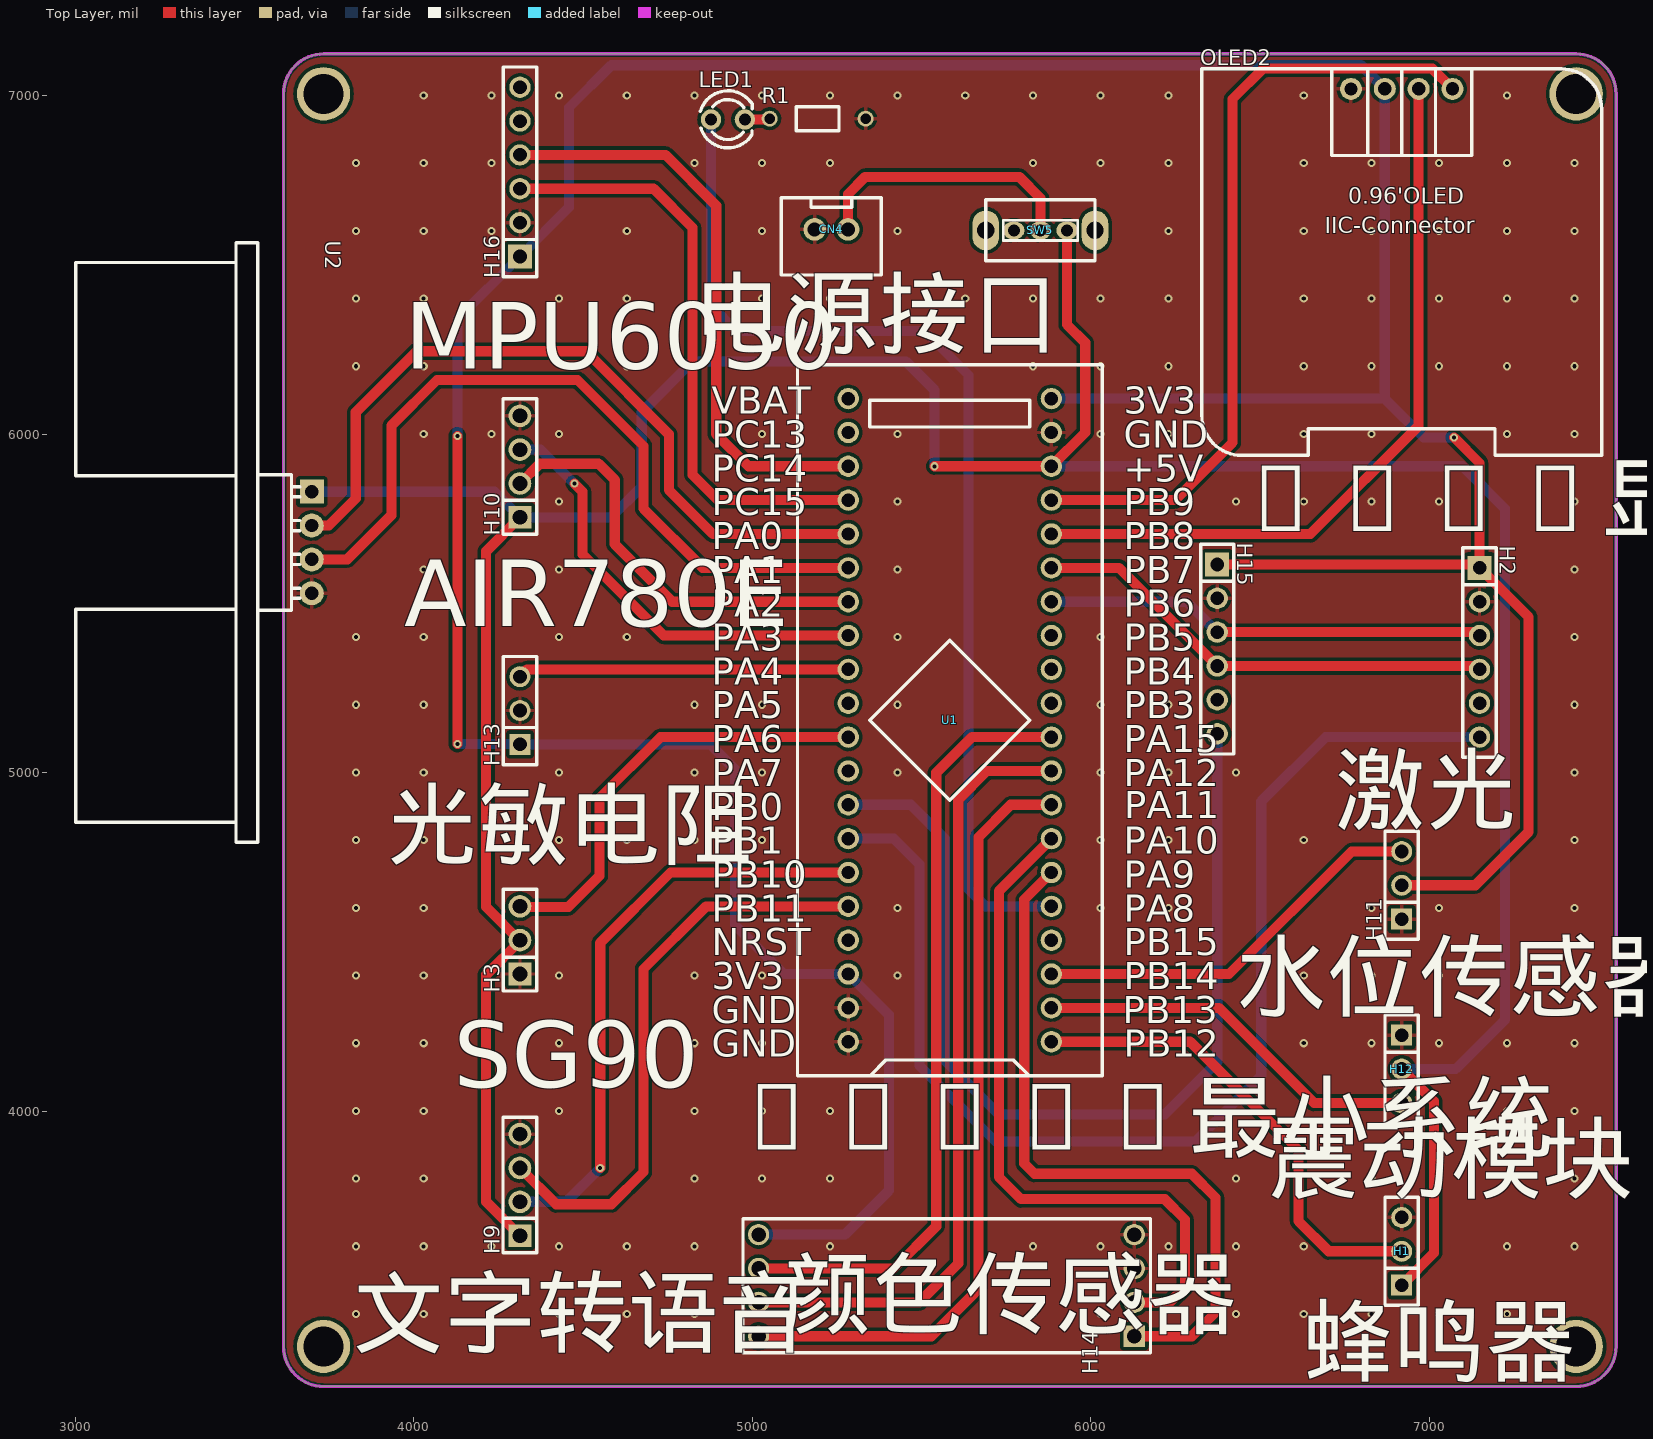
[diagram p0: Top Layer view]
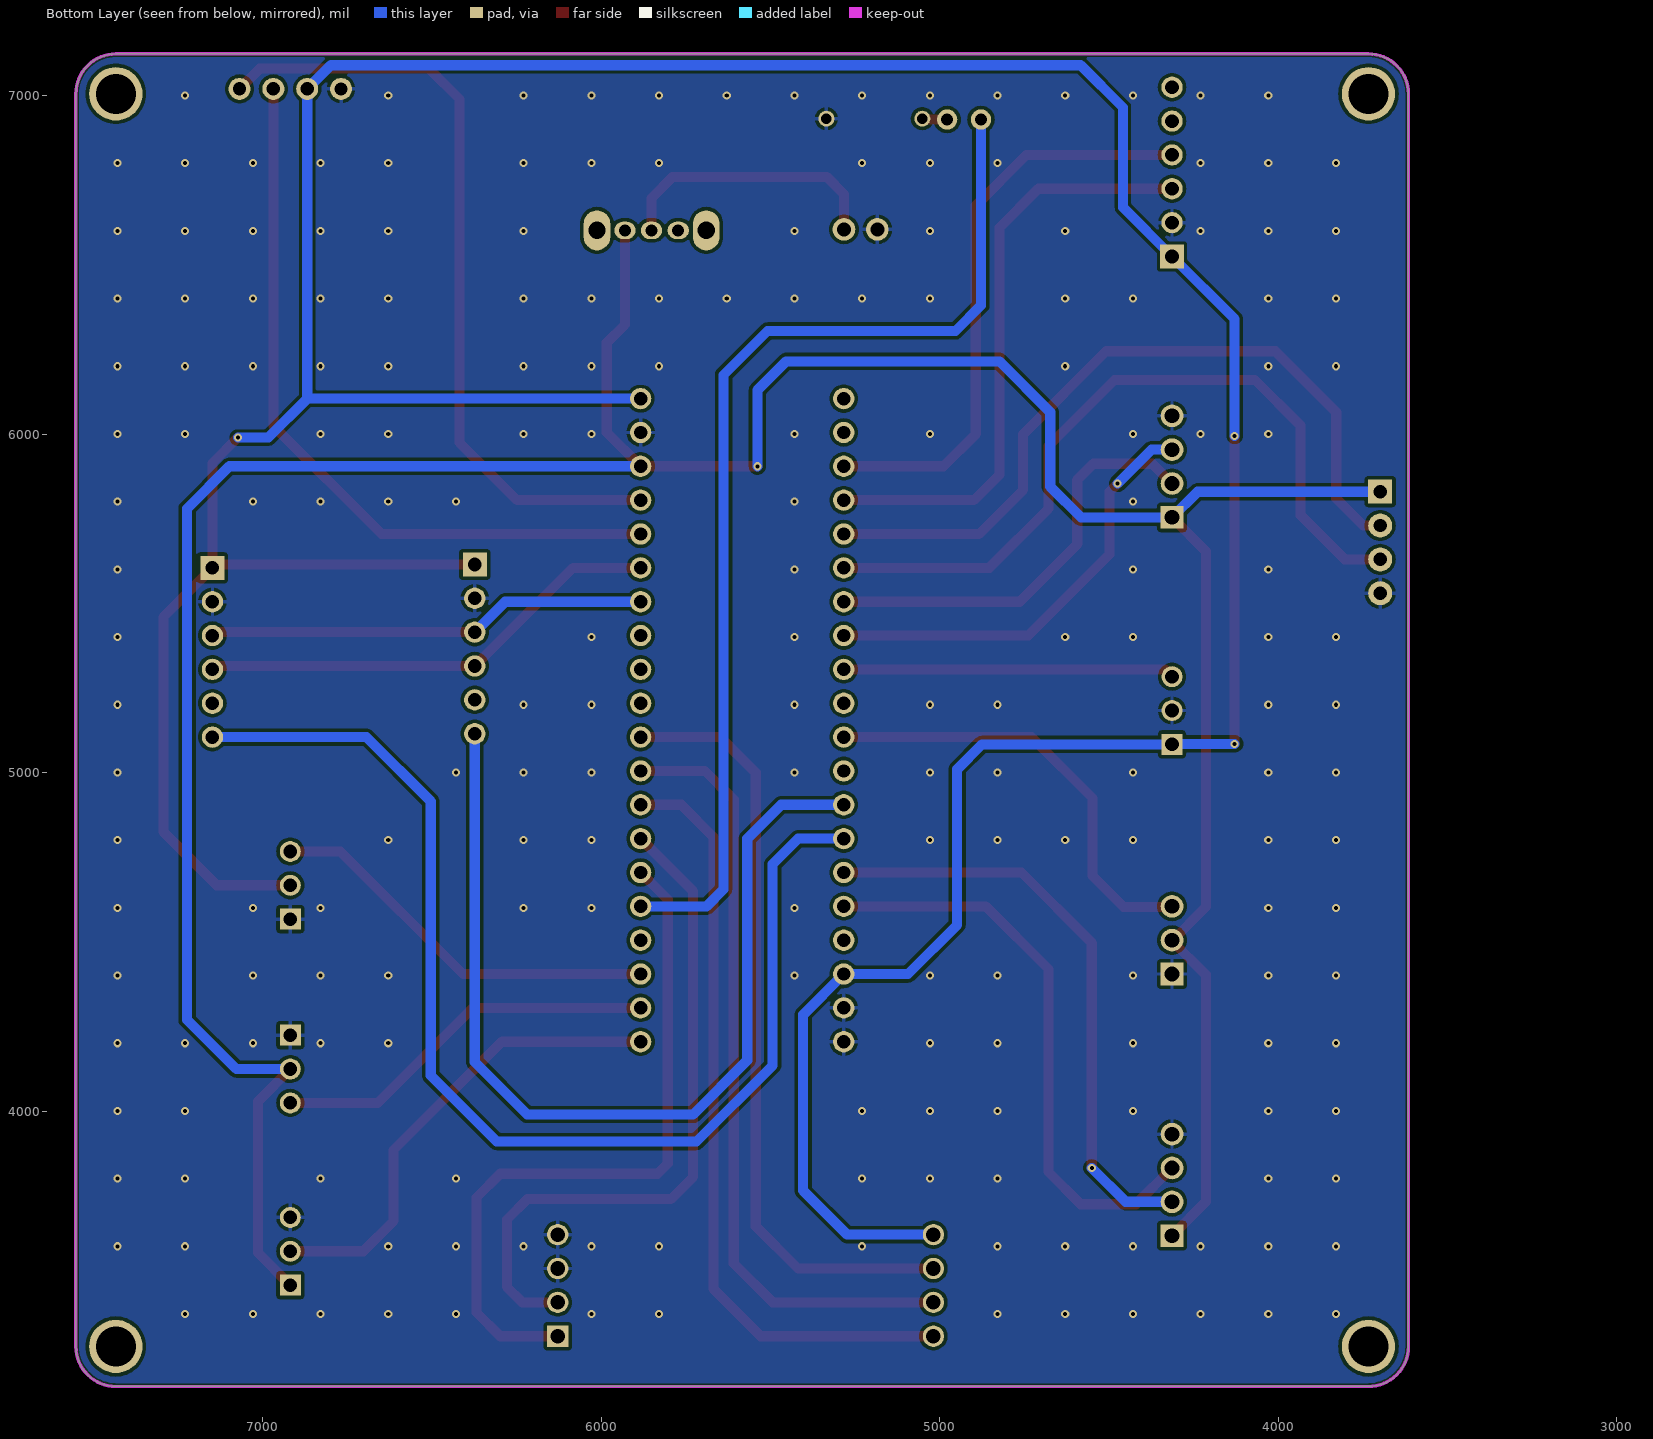
[diagram p1: Bottom Layer view, seen from below]
# Altium PCB MISC51292.pcbdoc
Units mil, origin at the board's own origin, x right, y up, seen from the top; angles counter-clockwise.
Board outline 3937.01 x 3937.01 mil, 2 copper layers (Top Layer, Bottom Layer), stack 62.206 mil thick; 18 components, 39 nets, 112 pads, 202 vias.

## Layer stack, top to bottom
Top Solder Mask Layer: solder mask 0.394, Dk 3.3
Top Layer: signal copper 1.379
Dielectric1: surface 59.449, FR4, Dk 4.5
Bottom Layer: signal copper 1.378
Bottom Solder Mask Layer: solder mask 0.394, Dk 3.3

## Board outline
3733.82,7123.5 ccw(c3733.82,7005.39) 3615.71,7005.39 3615.71,3304.61 ccw(c3733.82,3304.61) 3733.82,3186.5 7434.61,3186.5 ccw(c7434.61,3304.61) 7552.72,3304.61 7552.72,7005.39 ccw(c7434.61,7005.39) 7434.61,7123.5 3733.82,7123.5

## Design rules (kind name [scope] priority, off if disabled: settings)
BoardOutlineClearance copperThickness2oz_1 [All] p2 off: genericclearance=7.99 ignorepadtopadclearanceinfootprint=FALSE except(0: Arc-SplitContinuation Track-SplitContinuation SMDPad-SplitContinuation THPad-SplitContinuation Via-SplitContinuation Fill-SplitContinuation Region-SplitContinuation Poly-SplitContinuation Text-SplitContinuation Hole-SplitContinuation; 5.98: Arc-CutoutEdge Track-CutoutEdge SMDPad-CutoutEdge THPad-CutoutEdge Via-CutoutEdge Text-CutoutEdge; 6.9: Hole-OutlineEdge Hole-CutoutEdge; 10: Poly-OutlineEdge Poly-CutoutEdge; 11.81: Arc-OutlineEdge Track-OutlineEdge SMDPad-OutlineEdge THPad-OutlineEdge Via-OutlineEdge Fill-OutlineEdge Region-OutlineEdge Text-OutlineEdge Fill-CutoutEdge Region-CutoutEdge)
BoardOutlineClearance Plane_innerPlane_1 [All] p4 off: genericclearance=4.02 ignorepadtopadclearanceinfootprint=FALSE except(0: Arc-SplitContinuation Track-SplitContinuation SMDPad-SplitContinuation THPad-SplitContinuation Via-SplitContinuation Fill-SplitContinuation Region-SplitContinuation Poly-SplitContinuation Text-SplitContinuation Hole-SplitContinuation; 5.98: Arc-CutoutEdge Track-CutoutEdge SMDPad-CutoutEdge THPad-CutoutEdge Via-CutoutEdge Text-CutoutEdge; 6.9: Hole-OutlineEdge Hole-CutoutEdge; 10: Poly-OutlineEdge Poly-CutoutEdge; 11.81: Arc-OutlineEdge Track-OutlineEdge SMDPad-OutlineEdge THPad-OutlineEdge Via-OutlineEdge Fill-OutlineEdge Region-OutlineEdge Text-OutlineEdge Fill-CutoutEdge Region-CutoutEdge)
BoardOutlineClearance Copper_copperRegion_1 [All] p6 off: genericclearance=4.02 ignorepadtopadclearanceinfootprint=FALSE except(0: Arc-SplitContinuation Track-SplitContinuation SMDPad-SplitContinuation THPad-SplitContinuation Via-SplitContinuation Fill-SplitContinuation Region-SplitContinuation Poly-SplitContinuation Text-SplitContinuation Hole-SplitContinuation; 5.98: Arc-CutoutEdge Track-CutoutEdge SMDPad-CutoutEdge THPad-CutoutEdge Via-CutoutEdge Text-CutoutEdge; 6.9: Hole-OutlineEdge Hole-CutoutEdge; 10: Poly-OutlineEdge Poly-CutoutEdge; 11.81: Arc-OutlineEdge Track-OutlineEdge SMDPad-OutlineEdge THPad-OutlineEdge Via-OutlineEdge Fill-OutlineEdge Region-OutlineEdge Text-OutlineEdge Fill-CutoutEdge Region-CutoutEdge)
BoardOutlineClearance Copper_copperRegion_copperThickness1oz_1 [All] p8 off: genericclearance=4.02 ignorepadtopadclearanceinfootprint=FALSE except(0: Arc-SplitContinuation Track-SplitContinuation SMDPad-SplitContinuation THPad-SplitContinuation Via-SplitContinuation Fill-SplitContinuation Region-SplitContinuation Poly-SplitContinuation Text-SplitContinuation Hole-SplitContinuation; 5.98: Arc-CutoutEdge Track-CutoutEdge SMDPad-CutoutEdge THPad-CutoutEdge Via-CutoutEdge Text-CutoutEdge; 6.9: Hole-OutlineEdge Hole-CutoutEdge; 10: Poly-OutlineEdge Poly-CutoutEdge; 11.81: Arc-OutlineEdge Track-OutlineEdge SMDPad-OutlineEdge THPad-OutlineEdge Via-OutlineEdge Fill-OutlineEdge Region-OutlineEdge Text-OutlineEdge Fill-CutoutEdge Region-CutoutEdge)
BoardOutlineClearance Copper_copperRegion_Copper_copperRegion_1 [All] p10 off: genericclearance=4.02 ignorepadtopadclearanceinfootprint=FALSE except(0: Arc-SplitContinuation Track-SplitContinuation SMDPad-SplitContinuation THPad-SplitContinuation Via-SplitContinuation Fill-SplitContinuation Region-SplitContinuation Poly-SplitContinuation Text-SplitContinuation Hole-SplitContinuation; 5.98: Arc-CutoutEdge Track-CutoutEdge SMDPad-CutoutEdge THPad-CutoutEdge Via-CutoutEdge Text-CutoutEdge; 6.9: Hole-OutlineEdge Hole-CutoutEdge; 10: Poly-OutlineEdge Poly-CutoutEdge; 11.81: Arc-OutlineEdge Track-OutlineEdge SMDPad-OutlineEdge THPad-OutlineEdge Via-OutlineEdge Fill-OutlineEdge Region-OutlineEdge Text-OutlineEdge Fill-CutoutEdge Region-CutoutEdge)
BoardOutlineClearance copperThickness1oz_1 [All] p12: genericclearance=4.02 ignorepadtopadclearanceinfootprint=FALSE except(0: Arc-SplitContinuation Track-SplitContinuation SMDPad-SplitContinuation THPad-SplitContinuation Via-SplitContinuation Fill-SplitContinuation Region-SplitContinuation Poly-SplitContinuation Text-SplitContinuation Hole-SplitContinuation; 5.98: Arc-CutoutEdge Track-CutoutEdge SMDPad-CutoutEdge THPad-CutoutEdge Via-CutoutEdge Text-CutoutEdge; 6.9: Hole-OutlineEdge Hole-CutoutEdge; 10: Poly-OutlineEdge Poly-CutoutEdge; 11.81: Arc-OutlineEdge Track-OutlineEdge SMDPad-OutlineEdge THPad-OutlineEdge Via-OutlineEdge Fill-OutlineEdge Region-OutlineEdge Text-OutlineEdge Fill-CutoutEdge Region-CutoutEdge)
Clearance copperThickness2oz [All] p1 off: gap=7.99 ignorepadtopadclearanceinfootprint=FALSE except(5.98: SMDPad-Track SMDPad-SMDPad THPad-Track SMDPad-THPad THPad-THPad Track-Via SMDPad-Via THPad-Via Via-Via Fill-SMDPad Region-SMDPad Fill-THPad Region-THPad Fill-Via Region-Via Fill-Fill Fill-Region Region-Region Arc-Track Arc-SMDPad Arc-THPad Arc-Via Fill-Arc Region-Arc Arc-Arc Text-Track SMDPad-Text Text-THPad Text-Via Fill-Text Region-Text Arc-Text Text-Text; 6.9: Hole-Track Hole-SMDPad Hole-THPad Hole-Via Fill-Hole Region-Hole Hole-Arc Hole-Text; 10: Poly-Track Poly-SMDPad Poly-THPad Poly-Via Poly-Fill Poly-Region Poly-Poly Poly-Arc Poly-Text Poly-Hole; 11.81: Fill-Track Region-Track)
Clearance Plane_innerPlane [All] p3 off: gap=4.02 ignorepadtopadclearanceinfootprint=FALSE except(5.98: SMDPad-Track SMDPad-SMDPad THPad-Track SMDPad-THPad THPad-THPad Track-Via SMDPad-Via THPad-Via Via-Via Fill-SMDPad Region-SMDPad Fill-THPad Region-THPad Fill-Via Region-Via Fill-Fill Fill-Region Region-Region Arc-Track Arc-SMDPad Arc-THPad Arc-Via Fill-Arc Region-Arc Arc-Arc Text-Track SMDPad-Text Text-THPad Text-Via Fill-Text Region-Text Arc-Text Text-Text; 6.9: Hole-Track Hole-SMDPad Hole-THPad Hole-Via Fill-Hole Region-Hole Hole-Arc Hole-Text; 10: Poly-Track Poly-SMDPad Poly-THPad Poly-Via Poly-Fill Poly-Region Poly-Poly Poly-Arc Poly-Text Poly-Hole; 11.81: Fill-Track Region-Track)
Clearance Copper_copperRegion [All] p5 off: gap=4.02 ignorepadtopadclearanceinfootprint=FALSE except(5.98: SMDPad-Track SMDPad-SMDPad THPad-Track SMDPad-THPad THPad-THPad Track-Via SMDPad-Via THPad-Via Via-Via Fill-SMDPad Region-SMDPad Fill-THPad Region-THPad Fill-Via Region-Via Fill-Fill Fill-Region Region-Region Arc-Track Arc-SMDPad Arc-THPad Arc-Via Fill-Arc Region-Arc Arc-Arc Text-Track SMDPad-Text Text-THPad Text-Via Fill-Text Region-Text Arc-Text Text-Text; 6.9: Hole-Track Hole-SMDPad Hole-THPad Hole-Via Fill-Hole Region-Hole Hole-Arc Hole-Text; 10: Poly-Track Poly-SMDPad Poly-THPad Poly-Via Poly-Fill Poly-Region Poly-Poly Poly-Arc Poly-Text Poly-Hole; 11.81: Fill-Track Region-Track)
Clearance Copper_copperRegion_copperThickness1oz [All] p7 off: gap=4.02 ignorepadtopadclearanceinfootprint=FALSE except(5.98: SMDPad-Track SMDPad-SMDPad THPad-Track SMDPad-THPad THPad-THPad Track-Via SMDPad-Via THPad-Via Via-Via Fill-SMDPad Region-SMDPad Fill-THPad Region-THPad Fill-Via Region-Via Fill-Fill Fill-Region Region-Region Arc-Track Arc-SMDPad Arc-THPad Arc-Via Fill-Arc Region-Arc Arc-Arc Text-Track SMDPad-Text Text-THPad Text-Via Fill-Text Region-Text Arc-Text Text-Text; 6.9: Hole-Track Hole-SMDPad Hole-THPad Hole-Via Fill-Hole Region-Hole Hole-Arc Hole-Text; 10: Poly-Track Poly-SMDPad Poly-THPad Poly-Via Poly-Fill Poly-Region Poly-Poly Poly-Arc Poly-Text Poly-Hole; 11.81: Fill-Track Region-Track)
Clearance Copper_copperRegion_Copper_copperRegion [All] p9 off: gap=4.02 ignorepadtopadclearanceinfootprint=FALSE except(5.98: SMDPad-Track SMDPad-SMDPad THPad-Track SMDPad-THPad THPad-THPad Track-Via SMDPad-Via THPad-Via Via-Via Fill-SMDPad Region-SMDPad Fill-THPad Region-THPad Fill-Via Region-Via Fill-Fill Fill-Region Region-Region Arc-Track Arc-SMDPad Arc-THPad Arc-Via Fill-Arc Region-Arc Arc-Arc Text-Track SMDPad-Text Text-THPad Text-Via Fill-Text Region-Text Arc-Text Text-Text; 6.9: Hole-Track Hole-SMDPad Hole-THPad Hole-Via Fill-Hole Region-Hole Hole-Arc Hole-Text; 10: Poly-Track Poly-SMDPad Poly-THPad Poly-Via Poly-Fill Poly-Region Poly-Poly Poly-Arc Poly-Text Poly-Hole; 11.81: Fill-Track Region-Track)
Clearance copperThickness1oz [All] p11: gap=4.02 ignorepadtopadclearanceinfootprint=FALSE except(5.98: SMDPad-Track SMDPad-SMDPad THPad-Track SMDPad-THPad THPad-THPad Track-Via SMDPad-Via THPad-Via Via-Via Fill-SMDPad Region-SMDPad Fill-THPad Region-THPad Fill-Via Region-Via Fill-Fill Fill-Region Region-Region Arc-Track Arc-SMDPad Arc-THPad Arc-Via Fill-Arc Region-Arc Arc-Arc Text-Track SMDPad-Text Text-THPad Text-Via Fill-Text Region-Text Arc-Text Text-Text; 6.9: Hole-Track Hole-SMDPad Hole-THPad Hole-Via Fill-Hole Region-Hole Hole-Arc Hole-Text; 10: Poly-Track Poly-SMDPad Poly-THPad Poly-Via Poly-Fill Poly-Region Poly-Poly Poly-Arc Poly-Text Poly-Hole; 11.81: Fill-Track Region-Track)
DiffPairsRouting differentialPair [All] p1: maxlimit=6 minlimit=6 mostfreqgap=6 toplayer_minwidth=5 toplayer_prefwidth=10 toplayer_maxwidth=100 toplayer_mingap=6 toplayer_prefgap=6 toplayer_maxgap=6 bottomlayer_minwidth=5 bottomlayer_prefwidth=10 bottomlayer_maxwidth=100 bottomlayer_mingap=6 bottomlayer_prefgap=6 bottomlayer_maxgap=6 maxuncoupledlength=10
HoleToHoleClearance otherClearance [All] p1: gap=11.81 allowstackedmicrovias=TRUE
Length netLength [All] p1: minlimit=0 maxlimit=0
PasteMaskExpansion pasteMaskExpansion [All] p1: expansion=0
PlaneConnect innerPlane [All] p1: planeconnectstyle=Relief reliefexpansion=20 reliefentries=4 reliefconductorwidth=10 reliefairgap=10
PolygonConnect copperRegion_copperThickness1oz [All] p1 off: connectstyle=Relief reliefconductorwidth=10 reliefentries=4 polygonreliefangle="90 Angle" airgapwidth=10 via.connectstyle=Relief via.reliefconductorwidth=10 via.reliefentries=4 via.polygonreliefangle="90 Angle" via.airgapwidth=10
PolygonConnect copperRegion_Copper_copperRegion [All] p2 off: connectstyle=Relief reliefconductorwidth=10 reliefentries=4 polygonreliefangle="90 Angle" airgapwidth=10 via.connectstyle=Relief via.reliefconductorwidth=10 via.reliefentries=4 via.polygonreliefangle="90 Angle" via.airgapwidth=10
PolygonConnect copperRegion [All] p3: connectstyle=Relief reliefconductorwidth=10 reliefentries=4 polygonreliefangle="90 Angle" airgapwidth=10 via.connectstyle=Relief via.reliefconductorwidth=10 via.reliefentries=4 via.polygonreliefangle="90 Angle" via.airgapwidth=10
RoutingVias viaSize [All] p1: holewidth=12.01 width=24.02 viastyle="Through Hole" minholewidth=11.81 minwidth=19.68 maxholewidth=248.03 maxwidth=393.7
SolderMaskExpansion solderMaskExpansion [IsVia] p1: expansion=-1000 istentingtop=TRUE
SolderMaskExpansion solderMaskExpansion [All] p2: expansion=2 istentingtop=FALSE
Width copperThickness2oz_2 [All] p1 off: maxlimit=100 minlimit=8 preferedwidth=10
Width copperThickness1oz_2 [All] p2: maxlimit=100 minlimit=5 preferedwidth=10

## Components (designator, comment, footprint, x,y, rotation, side; value= is the part's Value field where it differs from the comment)
CN4 "XH2.54*2P_直插" CONN-TH_2P-P2.50-XH2.54-2P 5234.21,6605 r0 top
H1 "" HDR-TH_3P-P2.54-V-F 6919.21,3585.94 r90 top
H2 "" HDR-TH_6P-P2.54-V-F 7149.21,5355 r270 top
H3 "" HDR-TH_3P-P2.54-V-M 4314.21,4505 r90 top
H9 "" HDR-TH_4P-P2.54-V-M 4314.21,3782.03 r90 top
H10 "" HDR-TH_4P-P2.54-V-M 4314.21,5904.22 r90 top
H11 "" HDR-TH_3P-P2.54-V-F 6919.21,4667.11 r90 top
H12 "" HDR-TH_3P-P2.54-V-F 6919.21,4124.29 r270 top
H13 "" HDR-TH_3P-P2.54-V-F 4314.21,5183.44 r90 top
H14 "" HDR-TH_8P-P2.54-V-F-R2-C4-S2.54-1 6129.21,3435 r90 top
H15 "" HDR-TH_6P-P2.54-V-F 6374.21,5365 r270 top
H16 "" HDR-TH_6P-P2.54-V-F 4314.21,6775 r90 top
LED1 "" LED_TH-3mm 4928.67,6929.51 r0 top
OLED2 "" 0.96OLED_4P 6919.21,7020 r0 top
R1 "100" Res_1/8W 5193.66,6929.51 r0 top
SW5 "" 拨动开关 5857.11,6602.05 r180 top
U1 "STM32F103C8T6-Card" CONN-TH_L53.3-W22.9_STM32F103C8T6-CARD 5584.21,5155 r90 top
U2 "HC-SR04" TH_HC-SR04V 3699.21,5680 r270 top

## Footprints (in the part's own frame and the unit in brackets; to place one, negate y for a bottom-side part, rotate by r counter-clockwise, add the part's x,y. Pads: shape width x height; smd on the part's side, far side on the other; paste and mask are expansions set on the pad)
0.96OLED_4P [mm]
  round 1.65 hole 1 copper offset 0,0: 1(-3.81,-0.001) 2(-1.27,0.002) 3(1.27,0.002) 4(3.81,0.002)
  silkscreen extent -15,-27.5 15,1.5
CONN-TH_2P-P2.50-XH2.54-2P [mm]
  round 1.7 hole 1.05 paste+0 mask+0.05: 1(1.25,0) 2(-1.25,0)
  silkscreen extent -3.75,-3.42 3.75,2.37
CONN-TH_L53.3-W22.9_STM32F103C8T6-CARD [mm]
  round 1.6 hole 1: 1(-24.13,-7.62) 2(-21.59,-7.62) 3(-19.05,-7.62) 4(-16.51,-7.62) 5(-13.97,-7.62) 6(-11.43,-7.62) 7(-8.89,-7.62) 8(-6.35,-7.62) 9(-3.81,-7.62) 10(-1.27,-7.62) 11(1.27,-7.62) 12(3.81,-7.62) 13(6.35,-7.62) 14(8.89,-7.62) 15(11.43,-7.62) 16(13.97,-7.62) 17(16.51,-7.62) 18(19.05,-7.62) 19(21.59,-7.62) 20(24.13,-7.62) 21(24.13,7.62) 22(21.59,7.62) 23(19.05,7.62) 24(16.51,7.62) 25(13.97,7.62) 26(11.43,7.62) 27(8.89,7.62) 28(6.35,7.62) 29(3.81,7.62) 30(1.27,7.62) 31(-1.27,7.62) 32(-3.81,7.62) 33(-6.35,7.62) 34(-8.89,7.62) 35(-11.43,7.62) 36(-13.97,7.62) 37(-16.51,7.62) 38(-19.05,7.62) 39(-21.59,7.62) 40(-24.13,7.62)
  silkscreen extent -26.67,-11.43 26.67,11.43
HDR-TH_3P-P2.54-V-F [mil]
  rect 62x62 hole 40.16: 1(-100,0)
  round 62 hole 40.16: 2(0,0) 3(100,0)
  silkscreen extent -160,-49 160,49
HDR-TH_3P-P2.54-V-M [mm]
  rect 1.7x1.7 hole 1.1: 1(-2.54,0)
  round 1.7 hole 1.1: 2(0,0) 3(2.54,0)
  silkscreen extent -3.81,-1.25 3.81,1.25
HDR-TH_4P-P2.54-V-M [mm]
  rect 1.7x1.7 hole 1.1: 1(-3.81,0)
  round 1.7 hole 1.1: 2(-1.27,0) 3(1.27,0) 4(3.81,0)
  silkscreen extent -5.08,-1.27 5.08,1.27
HDR-TH_6P-P2.54-V-F [mm]
  rect 1.8x1.8 hole 1.02: 1(-6.35,0)
  round 1.6 hole 1.02: 2(-3.81,0) 3(-1.27,0) 4(1.27,0) 5(3.81,0) 6(6.35,0)
  silkscreen extent -7.87,-1.25 7.87,1.25
HDR-TH_8P-P2.54-V-F-R2-C4-S2.54-1 [mm]
  rect 1.6x1.6 hole 1.1: 1(-2.54,0)
  round 1.6 hole 1.1: 2(-2.54,28.194) 3(0,0) 4(0,28.194) 5(2.54,0) 6(2.54,28.194) 7(5.08,0) 8(5.08,28.194)
  silkscreen extent -3.78,-1.21 6.29,29.36
LED_TH-3mm [mil]
  round 60 hole 36 paste+0 mask+2: 1(-50,0) 2(50,0)
  silkscreen extent -81,-84 72,85
Res_1/8W [mil]
  round 47.2 hole 31.5 paste+0 mask+2: 1(-141.7,2.48) 2(141.7,2.48)
  silkscreen extent -63,-33 63,38
TH_HC-SR04V [mm]
  rect 1.8x1.8 hole 1.001: 1(-3.81,0)
  round 1.8 hole 1.001: 2(-1.27,0) 3(1.27,0) 4(3.81,0)
  silkscreen extent -22.5,-17.7 22.5,-0.89
拨动开关 [mil]
  oval 63x51.2 hole 35.4 paste+0 mask+2: 1(-73.4,0) 2(5,0) 3(84,0)
  oval 78.7x118.1 hole 51.2 paste+0 mask+2: 4(166.7,0) 5(-156.1,0)
  silkscreen extent -156,-90 167,90

## Free pads (board coordinates)
  round 157.48 hole 118.11: 1(3733.82,7005.39) 1(3733.82,3304.61) 1(7434.61,7005.39) 1(7434.61,3304.61)

## Via types
v1: diameter 24.02, hole 12, Top Layer to Bottom Layer, 202 vias

## Nets (pads, with @x,y where several pads share a name; then routed paths per layer and width w, separated by ;. In a path a pad name is that pad's centre, name@x,y a point inside that pad or via, vN(x,y) a via of type N, cw(c..) or ccw(c..) an arc to the next point about the centre after c; other vN are vias at no path point)
$1N17118: CN4.1 SW5.2 | length 815
  Top Layer w30: CN4.1 5283.43,6709.22 5334.21,6760 5789.21,6760 5852.11,6697.1 SW5.2
$1N17160: LED1.2 R1.1 | length 74.3
  Top Layer w30: LED1.2 5049.48,6929.51 R1.1
+5V: H1.1 H3.2 H9.1 H10.1 H12.2 SW5.1 U1.18 U2.1 | length 9829.1
  Top Layer w30: H9.1 4214.21,3732.03 4214.21,4402.82 4314.21,4502.82 4214.21,4602.82 4214.21,5654.22 H10.1 ; v1(5539.21,5905) U1.18 5984.21,6005 5984.21,6270 5930.51,6323.7 SW5.1 ; H1.1 7014.21,3580.95 7014.21,4029.29 H12.2
  Bottom Layer w30: U2.1 4238.43,5830 H10.1 4583.43,5754.22 4674.21,5845 4674.21,6065 4824.21,6215 5454.21,6215 5539.21,6130 v1(5539.21,5905) ; U1.18 7099.21,5905 7224.21,5780 7224.21,4270 7078.5,4124.29 H12.2
GND: CN4.2 H1.3 H2.2 H3.1 H9.4 H10.4 H11.1 H12.1 H13.2 H14.5 H14.7 H15.2 H16.2 OLED2.1 R1.2 U1.19 U1.39 U1.40 U2.4
  other v1: 3829.81,3400.6 4029.81,3400.6 4229.81,3400.6 4429.81,3400.6 4629.81,3400.6 4829.81,3400.6 5829.81,3400.6 6029.81,3400.6 6429.81,3400.6 6629.81,3400.6 6829.81,3400.6 7029.81,3400.6 7229.81,3400.6 3829.81,3600.6 4029.81,3600.6 4229.81,3600.6 4429.81,3600.6 4629.81,3600.6 4829.81,3600.6 5229.81,3600.6 5829.81,3600.6 6029.81,3600.6 6229.81,3600.6 6429.81,3600.6 6629.81,3600.6 7229.81,3600.6 7429.81,3600.6 3829.81,3800.6 4029.81,3800.6 4829.81,3800.6 5029.81,3800.6 5229.81,3800.6 6429.81,3800.6 6829.81,3800.6 7229.81,3800.6 7429.81,3800.6 3829.81,4000.6 4029.81,4000.6 4429.81,4000.6 4829.81,4000.6 5029.81,4000.6 5229.81,4000.6 7229.81,4000.6 7429.81,4000.6 3829.81,4200.6 4029.81,4200.6 4429.81,4200.6 4829.81,4200.6 5029.81,4200.6 6629.81,4200.6 6829.81,4200.6 7029.81,4200.6 7229.81,4200.6 7429.81,4200.6 3829.81,4400.6 4029.81,4400.6 4429.81,4400.6 4829.81,4400.6 5029.81,4400.6 5429.81,4400.6 6629.81,4400.6 6829.81,4400.6 7029.81,4400.6 7429.81,4400.6 3829.81,4600.6 4029.81,4600.6 5429.81,4600.6 6029.81,4600.6 6229.81,4600.6 6829.81,4600.6 7029.81,4600.6 7429.81,4600.6 3829.81,4800.6 4029.81,4800.6 4429.81,4800.6 4629.81,4800.6 4829.81,4800.6 5029.81,4800.6 6029.81,4800.6 6229.81,4800.6 6629.81,4800.6 7429.81,4800.6 3829.81,5000.6 4029.81,5000.6 4429.81,5000.6 4829.81,5000.6 5029.81,5000.6 5429.81,5000.6 6029.81,5000.6 6229.81,5000.6 6429.81,5000.6 7429.81,5000.6 3829.81,5200.6 4029.81,5200.6 4829.81,5200.6 5029.81,5200.6 5429.81,5200.6 6029.81,5200.6 6229.81,5200.6 7429.81,5200.6 3829.81,5400.6 4029.81,5400.6 4429.81,5400.6 4629.81,5400.6 5429.81,5400.6 6029.81,5400.6 7429.81,5400.6 4029.81,5600.6 4429.81,5600.6 5429.81,5600.6 7429.81,5600.6 4429.81,5800.6 5429.81,5800.6 6429.81,5800.6 6629.81,5800.6 6829.81,5800.6 7029.81,5800.6 7429.81,5800.6 4029.81,6000.6 4229.81,6000.6 4429.81,6000.6 5029.81,6000.6 5429.81,6000.6 6029.81,6000.6 6229.81,6000.6 6629.81,6000.6 6829.81,6000.6 7229.81,6000.6 7429.81,6000.6 3829.81,6200.6 4029.81,6200.6 4629.81,6200.6 5829.81,6200.6 6029.81,6200.6 6229.81,6200.6 6629.81,6200.6 6829.81,6200.6 7029.81,6200.6 7229.81,6200.6 7429.81,6200.6 3829.81,6400.6 4029.81,6400.6 4429.81,6400.6 4629.81,6400.6 5029.81,6400.6 5229.81,6400.6 5429.81,6400.6 5629.81,6400.6 5829.81,6400.6 6029.81,6400.6 6229.81,6400.6 6629.81,6400.6 6829.81,6400.6 7029.81,6400.6 7229.81,6400.6 7429.81,6400.6 3829.81,6600.6 4029.81,6600.6 4229.81,6600.6 4629.81,6600.6 5029.81,6600.6 5429.81,6600.6 6229.81,6600.6 6629.81,6600.6 6829.81,6600.6 7029.81,6600.6 7229.81,6600.6 7429.81,6600.6 3829.81,6800.6 4029.81,6800.6 4229.81,6800.6 4829.81,6800.6 5029.81,6800.6 5229.81,6800.6 5829.81,6800.6 6029.81,6800.6 6229.81,6800.6 6629.81,6800.6 6829.81,6800.6 7029.81,6800.6 7229.81,6800.6 7429.81,6800.6 4029.81,7000.6 4229.81,7000.6 4429.81,7000.6 4629.81,7000.6 4829.81,7000.6 5029.81,7000.6 5229.81,7000.6 5429.81,7000.6 5629.81,7000.6 5829.81,7000.6 6029.81,7000.6 6229.81,7000.6 6629.81,7000.6 7229.81,7000.6
NRST: U1.37
PA0: U1.25 U2.2 | length 2268
  Top Layer w30: U2.2 3749.21,5730 3829.21,5810 3829.21,6065 4009.21,6245 4509.21,6245 4754.21,6000 4754.21,5835 4884.21,5705 U1.25
PA1: U1.26 U2.3 | length 2298
  Top Layer w30: U2.3 3804.21,5630 3934.21,5760 3934.21,6025 4069.21,6160 4484.21,6160 4679.21,5965 4679.21,5780 4854.21,5605 U1.26
PA2: H10.2 U1.27 | length 1274.2
  Top Layer w30: H10.2 4372.49,5912.5 4546.71,5912.5 4594.21,5865 4594.21,5675 4764.21,5505 U1.27
PA3: H10.3 U1.28 | length 1305.9
  Top Layer w30: v1(4474.99,5854.22) 4499.21,5830 4499.21,5645 4739.21,5405 U1.28
  Bottom Layer w30: H10.3 4374.99,5954.22 v1(4474.99,5854.22)
PA4: H13.3 U1.29 | length 978.9
  Top Layer w30: H13.3 4335.78,5305 U1.29
PA5: U1.30
PA6: H3.3 U1.31 | length 1312.7
  Top Layer w30: H3.3@4314.21,4602.82 4457.03,4602.82 4549.21,4695 4549.21,4925 4729.21,5105 U1.31
PA7: U1.32
PA8: LED1.1 U1.5 | length 3180.4
  Bottom Layer w30: LED1.1 4878.67,6380.54 4954.21,6305 5509.21,6305 5639.21,6175 5639.21,4655 5689.21,4605 U1.5
PA9: H14.1 U1.6 | length 2108.6
  Top Layer w30: U1.6 5804.21,4625 5804.21,3845 5834.21,3815 6299.21,3815 6369.21,3745 6369.21,3405 6299.21,3335 H14.1
PA10: H14.3 U1.7 | length 2034.3
  Top Layer w30: U1.7 5729.21,4650 5729.21,3805.51 5794.72,3740 6219.21,3740 6279.21,3680 6279.21,3480 6234.21,3435 H14.3
PA11: H14.2 U1.8 | length 2297.3
  Top Layer w30: H14.2 5529.21,3335 5669.21,3475 5669.21,4810 5764.21,4905 U1.8
PA12: H14.4 U1.9 | length 2317.8
  Top Layer w30: H14.4 5494.21,3435 5609.21,3550 5609.21,4920 5694.21,5005 U1.9
PA15: H14.6 U1.10 | length 2300.3
  Top Layer w30: H14.6 5419.21,3535 5544.21,3660 5544.21,5000 5649.21,5105 U1.10
PB0: H15.6 U1.33 | length 2886.9
  Bottom Layer w30: U1.33 5469.21,4905 5569.21,4805 5569.21,4150 5729.21,3990 6219.21,3990 6374.21,4145 H15.6
PB1: H2.6 U1.34 | length 3553.7
  Bottom Layer w30: U1.34 5419.21,4805 5494.21,4730 5494.21,4135 5719.21,3910 6309.21,3910 6504.21,4105 6504.21,4915 6694.21,5105 H2.6
PB3: U1.11
PB4: U1.12
PB5: U1.13
PB6: H2.3 H15.3 U1.14 | length 1306.4
  Top Layer w30: H15.3 7139.21,5415 H2.3
  Bottom Layer w30: U1.14 6284.21,5505 H15.3
PB7: H2.4 H15.4 U1.15 | length 1389.3
  Top Layer w30: U1.15 6084.21,5605 H15.4 7139.21,5315 H2.4
PB8: OLED2.3 U1.16 | length 2212.6
  Top Layer w30: U1.16 6649.21,5705 6969.21,6025 OLED2.3@6969.21,7020.05
PB9: OLED2.4 U1.17 | length 2332.5
  Top Layer w30: U1.17 6249.21,5805 6419.21,5975 6419.21,6990 6509.21,7080 7009.26,7080 OLED2.4@7069.21,7020.05
PB10: H9.2 U1.35 | length 1762.6
  Top Layer w30: v1(4551.25,3832.03) 4551.25,4497.03 4759.21,4705 U1.35
  Bottom Layer w30: H9.2 4451.25,3732.03 v1(4551.25,3832.03)
PB11: H9.3 U1.36 | length 1730.3
  Top Layer w30: H9.3 4421.25,3725 4584.21,3725 4679.21,3820 4679.21,4420 4864.21,4605 U1.36
PB12: H1.2 U1.1 | length 1414.4
  Top Layer w30: U1.1 6294.21,4205 6614.21,3885 6614.21,3675 6703.27,3585.94 H1.2
PB13: H12.3 U1.2 | length 1151.3
  Top Layer w30: U1.2 6379.21,4305 6659.92,4024.29 H12.3
PB14: H11.3 U1.3 | length 1185
  Top Layer w30: U1.3 6409.21,4405 6771.32,4767.11 H11.3
PB15: U1.4
PC13: U1.22
PC14: H16.4 U1.23 | length 1746.5
  Top Layer w30: H16.4 4744.21,6825 4894.21,6675 4894.21,6000 4989.21,5905 U1.23
PC15: H16.3 U1.24 | length 1778.7
  Top Layer w30: H16.3 4709.21,6725 4824.21,6610 4824.21,5880 4899.21,5805 U1.24
VBAT: U1.21
VCC: H2.1 H11.2 H13.1 H14.8 H15.1 H16.1 OLED2.2 U1.20 U1.38 | length 11970.5
  Top Layer w30: v1(4129.21,5085) v1(4129.21,5995) ; H15.1 7139.21,5615 H2.1 ; H11.2 7136.32,4667.11 7294.21,4825 7294.21,5460 H2.1 ; v1(7074.21,5990) 7149.21,5915 H2.1
  Bottom Layer w30: v1(4129.21,5085) 4312.65,5085 H13.1 4875.77,5083.44 4949.21,5010 4949.21,4550 5094.21,4405 U1.38 5404.21,4285 5404.21,3765 5274.21,3635 H14.8 ; v1(4129.21,5995) 4129.21,6340 H16.1 4459.21,6670 4459.21,6965 4584.21,7090 6799.26,7090 6869.21,7020.05 6869.21,6105 ; U1.20 6869.21,6105 ; v1(7074.21,5990) 6984.21,5990 6869.21,6105
pads on no net: H2.5 H15.5 H16.5 H16.6 SW5.3 SW5.4 SW5.5

## Polygon pours and split planes (outlines as drawn)
GND on Bottom Layer (solid, remove dead copper, pour order 2): 3544.21,7245 3544.21,3080 7719.21,3080 7719.21,7245
GND on Top Layer (solid, remove dead copper, pour order 2): 3019.21,7415 3019.21,3000 7949.21,3000 7949.21,7415

## Keep-outs
Board Outline Layer:
  the board outline again, w10

## Silkscreen, mask and mechanical layers (free items; w line width, h text height)
Top Silkscreen Layer:
  text "电源接口" at 4832.09,6261.57 h196.85
  text "MPU6050" at 3973.9,6193.12 h196.85
  text "VBAT" at 4880.16,6060 h80
  text "3V3" at 6098.37,6060 h80
  text "PC13" at 4880.16,5960 h80
  text "GND" at 6098.37,5960 h80
  text "PC14" at 4880.16,5860 h80
  text "+5V" at 6098.37,5860 h80
  text "PC15" at 4880.16,5760 h80
  text "PB9" at 6098.37,5760 h80
  text "Oled显示器" at 6427.23,5712.52 h196.85
  text "PA0" at 4880.16,5660 h80
  text "PB8" at 6098.37,5660 h80
  text "PA1" at 4880.16,5560 h80
  text "PB7" at 6098.37,5560 h80
  text "PA2" at 4880.16,5460 h80
  text "PB6" at 6098.37,5460 h80
  text "AIR780E" at 3972.56,5432.18 h196.85
  text "PA3" at 4880.16,5360 h80
  text "PB5" at 6098.37,5360 h80
  text "PA4" at 4880.16,5260 h80
  text "PB4" at 6098.37,5260 h80
  text "PA5" at 4880.16,5160 h80
  text "PB3" at 6098.37,5160 h80
  text "PA6" at 4880.16,5060 h80
  text "PA15" at 6098.37,5060 h80
  text "PA7" at 4880.16,4960 h80
  text "PA12" at 6098.37,4960 h80
  text "PA11" at 6100.16,4865 h80
  text "PB0" at 4880.16,4860 h80
  text "激光" at 6722.06,4854.34 h196.85
  text "PB1" at 4880.16,4760 h80
  text "PA10" at 6098.37,4760 h80
  text "光敏电阻" at 3920.96,4751.56 h196.85
  text "PB10" at 4880.16,4660 h80
  text "PA9" at 6098.37,4660 h80
  text "PB11" at 4880.16,4560 h80
  text "PA8" at 6098.37,4560 h80
  text "NRST" at 4880.16,4460 h80
  text "PB15" at 6098.37,4460 h80
  text "3V3" at 4880.16,4360 h80
  text "PB14" at 6098.37,4360 h80
  text "水位传感器" at 6427.98,4302.64 h196.85
  text "GND" at 4880.16,4260 h80
  text "PB13" at 6095.16,4260 h80
  text "GND" at 4880.16,4160 h80
  text "PB12" at 6098.37,4160 h80
  text "SG90" at 4118.26,4070.94 h196.85
  text "STM32最小系统" at 4938.66,3886.57 h196.85
  text "震动模块" at 6523.31,3764.6 h196.85
  text "颜色传感器" at 5084.21,3365 h196.85
  text "文字转语音" at 3821.49,3310 h196.85
  text "蜂鸣器" at 6626.02,3224.16 h196.85